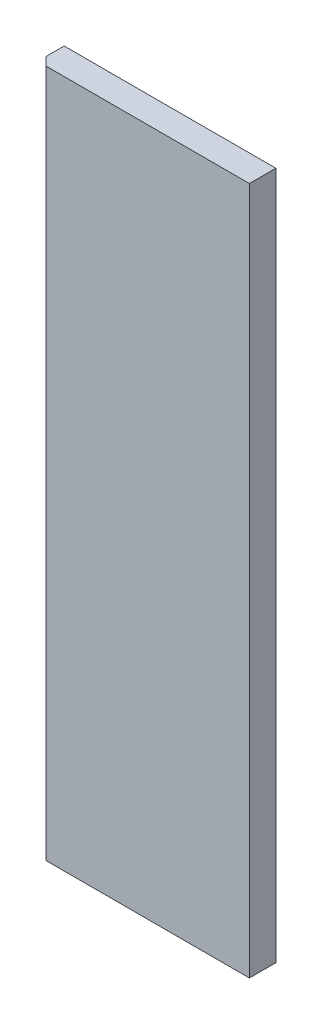
from build123d import *

# Parameters (mm, degrees)
SKETCH1_W           = 200
SKETCH1_H           = 650
BOSS_EXTRUDE1_DEPTH = 25
CHAMFER1_SIZE       = 8


with BuildPart() as part:
    # Sketch1 → Boss-Extrude1 (new body)
    with BuildSketch(Plane.XY):
        with Locations((100, 325)):
            Rectangle(SKETCH1_W, SKETCH1_H)
    extrude(amount=BOSS_EXTRUDE1_DEPTH)

    # Chamfer1
    chamfer1_edges = [part.edges().sort_by_distance(p)[0] for p in [
        (0, 325, 25),
    ]]
    chamfer(chamfer1_edges, length=CHAMFER1_SIZE)


solid = part.part
